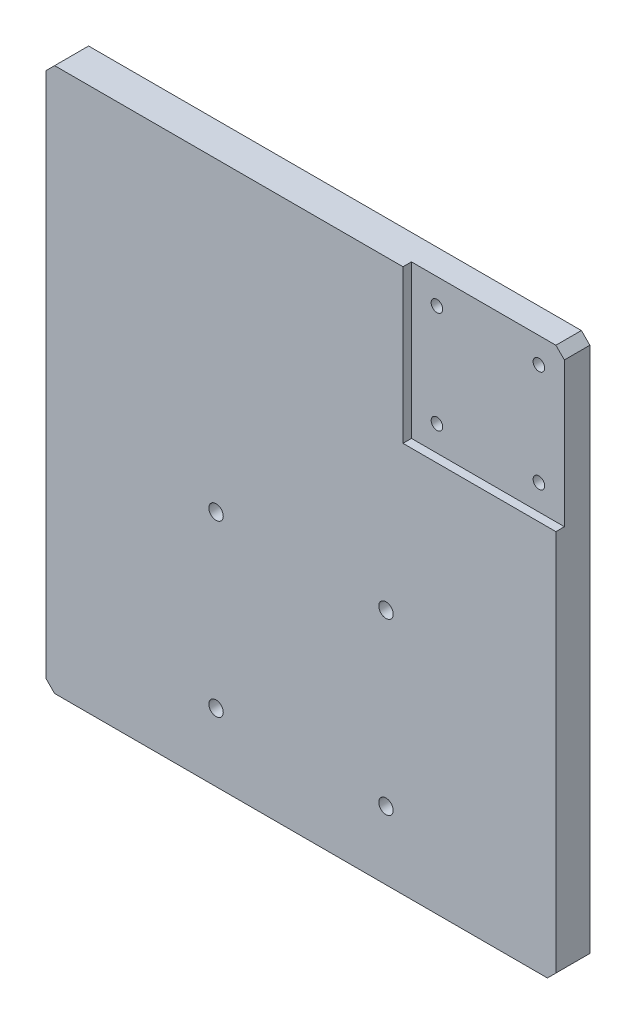
SolidWorks part; units mm, degrees
material "CuCrZr"
ref_plane "前视基准面" through (0, 0, 0) normal (0, 0, 1) x (1, 0, 0)
ref_plane "上视基准面" through (0, 0, 0) normal (0, 1, 0) x (1, 0, 0)
ref_plane "右视基准面" through (0, 0, 0) normal (1, 0, 0) x (0, 0, -1)
sketch "草图1" plane through (0, 0, 0) normal (0, 0, 1) x (1, 0, 0)
  line L5 (-150, -160) -> (150, -160)
  line L6 (-150, -160) -> (-150, 160)
  line L7 (-150, 160) -> (150, 160)
  line L8 (150, -160) -> (150, 160)
  line L9 (0, 160) -> (0, -160) construction
  line L10 (-150, 0) -> (150, 0) construction
  point P0 (0, 0)
  dimension "D1" = 300
  dimension "D2" = 320
extrude "凸台-拉伸1" add sketch "草图1" along normal mid plane 20
hole_wizard "M10 螺纹孔1" positions "草图4" profile "草图6" tap size "M10" standard "GB"
sketch "草图4" plane through (0, 0, 10) normal (0, 0, 1) x (1, 0, 0)
  line L1 (-50, -120) -> (50, -120) construction
  line L2 (-50, -120) -> (-50, -20) construction
  line L3 (-50, -20) -> (50, -20) construction
  line L4 (50, -120) -> (50, -20) construction
  line L5 (0, -20) -> (0, 20) construction
  line L6 (-50, 0) -> (50, 0) construction
  line L9 (-150, -160) -> (150, -160) construction
  point P3 (50, -20)
  point P202 (-50, -120)
  point P203 (-50, -20)
  point P204 (50, -120)
  dimension "D1" = 100
  dimension "D2" = 100
  dimension "D3" = 40
sketch "草图6" plane through (50, -20, 10) normal (1, 0, 0) x (0, -1, 0)
  line L0 (0, 0) -> (0, 17.5537)
  line L1 (0, 17.5537) -> (4.25, 15)
  line L2 (4.25, 15) -> (4.25, 0)
  line L5 (4.25, 0) -> (0, 0)
  line L10 (0, 17.5537) -> (-4.25, 15) construction
  line L11 (0, -6.35) -> (0, 107.95) construction
  dimension "螺纹孔钻头直径" = 8.5
  dimension "螺纹孔钻头深度" = 15
  dimension "导头角度" = 118
cosmetic thread "孔螺蚊线1"
cosmetic thread "孔螺蚊线2"
cosmetic thread "孔螺蚊线3"
cosmetic thread "孔螺蚊线4"
sketch "草图7" plane through (0, 0, 10) normal (0, 0, 1) x (1, 0, 0)
  line L0 (150, -160) -> (150, 160) construction
  line L2 (150, 70) -> (60, 70)
  line L3 (0, 160) -> (0, -160) construction
  line L8 (150, 160) -> (-150, 160) construction
  line L9 (-150, -160) -> (150, -160) construction
  line L10 (150, 70) -> (150, 160)
  line L11 (150, 160) -> (60, 160)
  line L12 (60, 70) -> (60, 160)
  dimension "D1" = 0
  dimension "D5" = 90
  dimension "D6" = 90
extrude "切除-拉伸1" cut sketch "草图7" against normal blind 5
hole_wizard "M8 螺纹孔1" positions "草图8" profile "草图10" tap size "M8" standard "GB"
sketch "草图8" plane through (0, 0, 5) normal (0, 0, 1) x (1, 0, 0)
  line L0 (60, 115) -> (150, 115) construction
  line L1 (60, 160) -> (60, 70) construction
  line L2 (150, 70) -> (150, 160) construction
  line L4 (75, 85) -> (135, 85) construction
  line L5 (75, 85) -> (75, 145) construction
  line L6 (75, 145) -> (135, 145) construction
  line L7 (135, 85) -> (135, 145) construction
  line L8 (105, 145) -> (105, 85) construction
  line L9 (75, 115) -> (135, 115) construction
  point P191 (75, 85)
  point P192 (75, 145)
  point P193 (135, 85)
  point P203 (135, 145)
  dimension "D1" = 60
  dimension "D2" = 60
  dimension "D3" = 15
sketch "草图10" plane through (135, 145, 5) normal (1, 0, 0) x (0, -1, 0)
  line L0 (0, 0) -> (0, 12.0429)
  line L1 (0, 12.0429) -> (3.4, 10)
  line L2 (3.4, 10) -> (3.4, 0)
  line L5 (3.4, 0) -> (0, 0)
  line L10 (0, 12.0429) -> (-3.4, 10) construction
  line L11 (0, -6.35) -> (0, 107.95) construction
  dimension "螺纹孔钻头直径" = 6.8
  dimension "螺纹孔钻头深度" = 10
  dimension "导头角度" = 118
cosmetic thread "孔螺蚊线5"
cosmetic thread "孔螺蚊线6"
cosmetic thread "孔螺蚊线7"
cosmetic thread "孔螺蚊线8"
chamfer "倒角1" distance 5 angle 45 4 edges at (150, 160, -2.5) (150, -160, 0) (-150, 160, 0) (-150, -160, 0)
